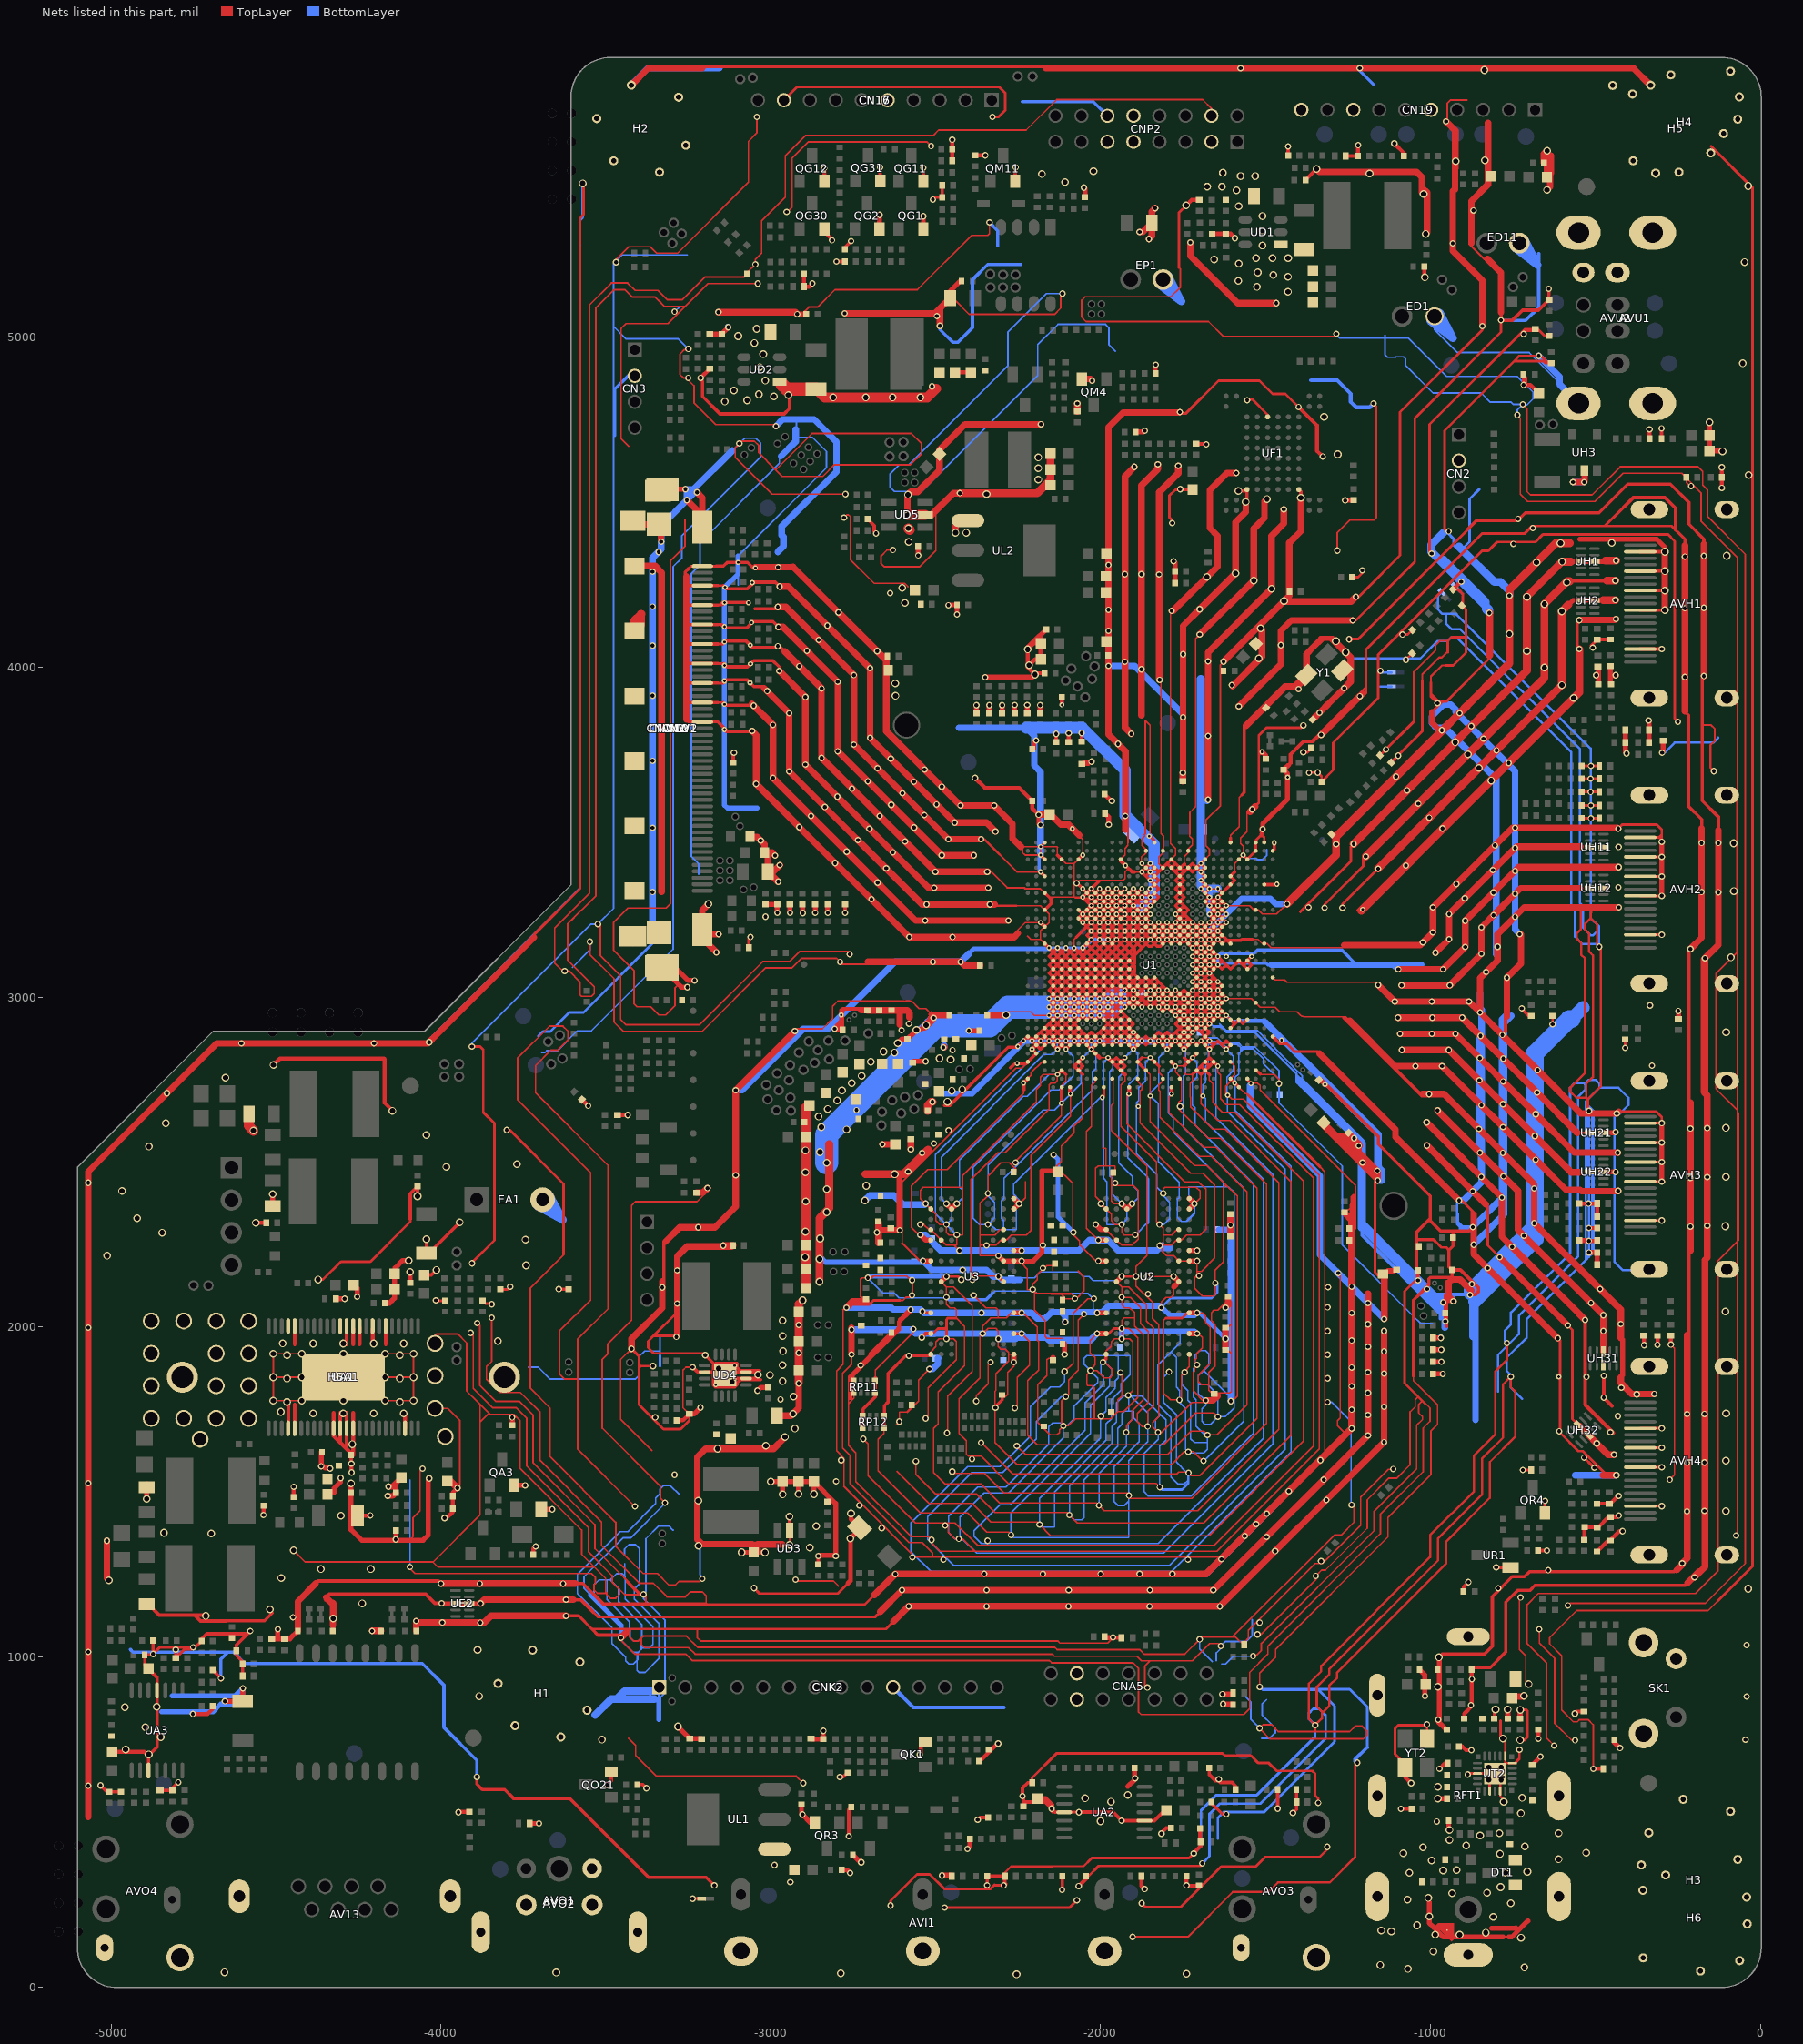
[diagram p0: the nets of this part, all layers, seen from the top]
# Altium PCB MISC86290.PcbDoc (part 18 of 31)
Units mil, origin at the board's own origin, x right, y up, seen from the top; angles counter-clockwise.
Board outline 5104.71 x 5851.49 mil, 2 copper layers (TopLayer, BottomLayer), stack 61.855 mil thick; 1026 components, 667 nets, 4280 pads, 2294 vias.

## Via types
v1: diameter 19.68, hole 11.81, TopLayer to BottomLayer, tented both sides, 1189 vias
v2: diameter 19.68/19.68 (per signal layer), hole 11.81, TopLayer to BottomLayer, tented both sides, 366 vias
v3: diameter 15.75, hole 7.87, TopLayer to BottomLayer, tented both sides, 348 vias
v4: diameter 23.62, hole 15.75, TopLayer to BottomLayer, tented both sides, 309 vias
v5: diameter 15.75/15.75 (per signal layer), hole 7.87, TopLayer to BottomLayer, tented both sides, 59 vias
v6: diameter 24/24 (per signal layer), hole 16, TopLayer to BottomLayer, tented both sides, 23 vias

## Nets (pads, with @x,y where several pads share a name; then routed paths per layer and width w, separated by ;. In a path a pad name is that pad's centre, name@x,y a point inside that pad or via, vN(x,y) a via of type N, cw(c..) or ccw(c..) an arc to the next point about the centre after c; other vN are vias at no path point) (continued)
GND: (continued)
  TopLayer w10: U1.W10@-1708.98,3187.6 v3(-1696.18,3174.8) U1.V9@-1683.39,3162.01 v3(-1670.59,3149.21) U1.U8@-1657.8,3136.42 ; -1696.18,2790.94 U1.C9@-1683.39,2778.15 ; -1696.18,2790.94 U1.D9@-1683.39,2803.74 ; v3(-1696.18,2867.72) U1.F9@-1683.39,2854.92 ; v3(-1696.18,2867.72) -1670.59,2893.31 U1.H9@-1683.39,2906.1 ; -1696.18,2893.31 U1.G9@-1683.39,2880.51 v3(-1670.59,2867.72) ; -1696.18,2893.31 U1.H9@-1683.39,2906.1 ; v3(-1696.18,2918.9) U1.H9@-1683.39,2906.1 ; v3(-1696.18,2918.9) U1.J9@-1683.39,2931.69 ; v3(-1696.18,2944.49) U1.J9@-1683.39,2931.69 ; v3(-1696.18,2944.49) -1683.39,2957.28 ; v3(-1696.18,2970.08) -1683.39,2957.28 ; v3(-1696.18,2970.08) U1.L9@-1683.39,2982.87 v3(-1670.59,2995.67) -1657.8,3008.46 v3(-1645,3021.26) U1.N7@-1632.2,3034.06 v3(-1645,3046.85) ; U1.C9@-1683.39,2778.15 -1670.59,2790.94 ; U1.D9@-1683.39,2803.74 -1670.59,2790.94 ; U1.D9@-1683.39,2803.74 -1670.59,2816.54 U1.D8@-1657.8,2803.74 ; U1.F9@-1683.39,2854.92 v5(-1670.59,2842.13) -1657.8,2854.92 ; U1.F9@-1683.39,2854.92 v3(-1670.59,2867.72) ; U1.H9@-1683.39,2906.1 v3(-1670.59,2918.9) ; U1.J9@-1683.39,2931.69 v3(-1670.59,2918.9) ; U1.J9@-1683.39,2931.69 v3(-1670.59,2944.49) ; -1683.39,2957.28 v3(-1670.59,2944.49) ; -1683.39,2957.28 v3(-1670.59,2970.08) U1.L8@-1657.8,2982.87 v3(-1645,2995.67) U1.M7@-1632.2,3008.46 ; U1.Y9@-1683.39,3213.19 v3(-1670.59,3225.98) ; U1.Y9@-1683.39,3213.19 v3(-1670.59,3200.39) ; U1.AD9@-1683.39,3315.55 v3(-1670.59,3302.76) ; -1670.59,2790.94 U1.D8@-1657.8,2803.74 ; v3(-1670.59,2867.72) -1657.8,2854.92 ; v3(-1670.59,2918.9) U1.J8@-1657.8,2931.69 ; v3(-1670.59,2944.49) U1.K8@-1657.8,2957.28 v3(-1645,2970.08) U1.L7@-1632.2,2982.87 ; v3(-1670.59,2944.49) U1.J8@-1657.8,2931.69 ; v3(-1670.59,3200.39) U1.Y8@-1657.8,3213.19 ; v3(-1670.59,3200.39) U1.W8@-1657.8,3187.6 v3(-1645,3174.8) U1.V7@-1632.2,3162.01 -1619.41,3174.8 ; v3(-1670.59,3225.98) U1.AA8@-1657.8,3238.78 ; v3(-1670.59,3225.98) U1.Y8@-1657.8,3213.19 ; v3(-1670.59,3277.17) U1.AC9@-1683.39,3289.96 v3(-1670.59,3302.76) ; v3(-1670.59,3277.17) v3(-1645,3251.57) ; v3(-1670.59,3277.17) U1.AC8@-1657.8,3289.96 ; v3(-1670.59,3302.76) U1.AC8@-1657.8,3289.96 ; -1657.8,2854.92 -1645,2867.72 -1632.52,2855.24 ; -1657.8,3059.65 v3(-1645,3046.85) ; -1657.8,3059.65 v3(-1721.77,3123.62) U1.Y7@-1632.2,3213.19 ; U1.U8@-1657.8,3136.42 v3(-1721.77,3072.44) U1.L7@-1632.2,2982.87 ; U1.U8@-1657.8,3136.42 v3(-1645,3123.62) ; U1.Y8@-1657.8,3213.19 U1.AA7@-1632.2,3238.78 ; U1.Y8@-1657.8,3213.19 v3(-1645,3200.39) U1.W7@-1632.2,3187.6 ; U1.AA8@-1657.8,3238.78 v3(-1670.59,3251.57) U1.AB8@-1657.8,3264.37 v3(-1645,3277.17) ; U1.AA8@-1657.8,3238.78 v3(-1645,3225.98) U1.Y7@-1632.2,3213.19 ; U1.AA8@-1657.8,3238.78 v3(-1645,3251.57) ; U1.AC8@-1657.8,3289.96 v3(-1645,3277.17) ; U1.AC8@-1657.8,3289.96 v3(-1645,3302.76) ; v3(-1645,3098.03) -1632.2,3085.24 -1619.41,3098.03 ; v3(-1645,3098.03) -1632.2,3110.83 ; v3(-1645,3123.62) -1632.2,3110.83 ; v3(-1645,3251.57) U1.AA7@-1632.2,3238.78 ; v3(-1645,3251.57) U1.AB7@-1632.2,3264.37 ; v3(-1645,3277.17) U1.AC7@-1632.2,3289.96 ; v3(-1645,3277.17) U1.AB7@-1632.2,3264.37 ; v3(-1645,3302.76) U1.AC7@-1632.2,3289.96 ; v3(-1645,3302.76) U1.AD7@-1632.2,3315.55 ; U1.L7@-1632.2,2982.87 -1619.34,2995.74 -1632.07,3008.46 U1.M7@-1632.2,3008.46 ; U1.M7@-1632.2,3008.46 v3(-1721.77,3098.03) U1.W7@-1632.2,3187.6 ; -1632.2,3110.83 -1619.41,3098.03 ; U1.W7@-1632.2,3187.6 -1619.41,3174.8 ; U1.Y7@-1632.2,3213.19 v3(-1619.41,3225.98) U1.AA7@-1632.2,3238.78 ; U1.AA7@-1632.2,3238.78 v3(-1619.41,3251.57) U1.AB7@-1632.2,3264.37 ; U1.AB7@-1632.2,3264.37 v3(-1619.41,3277.17) U1.AC7@-1632.2,3289.96 ; -1619.41,3098.03 -1606.61,3085.24 U1.T5@-1581.02,3110.83 -1568.23,3098.03 ; -1619.41,3174.8 -1617.01,3172.4 -1574.73,3172.4 ; -1568.23,3098.03 U1.T4@-1555.43,3110.83 ; -1568.23,3098.03 U1.R4@-1555.43,3085.24 -1542.64,3098.03 U1.T4@-1555.43,3110.83 ; -944.34,2220 -944.34,2182.31 RO2.1@-935.04,2173 ; -752.48,1243 -715.33,1243 -700.58,1257.75 v1@-638.28,1257.75 ; v1@-731,4450 -712.8,4468.2 -672.72,4468.2
  TopLayer w11: UA1.4@-4463.07,1692.73 pad.VIA5@-4463.07,1769.34 ; UA1.5@-4443.39,1692.73 -4443.39,1765.61 ; v1(-2066,529) -1962.59,529 v1(-1937,503.41) UA2.10@-1867.44,503.41 -1837.59,503.41 -1806,535 CO20.1@-1800.81,535 ; v1(-1816,464) -1816,466 -1801,481 CO21.1@-1786.73,481
  TopLayer w11.8: -4443.39,1947.88 UA1.44@-4443.39,1994.89 ; -4325.28,1739.74 -4325.28,1669.55 -4272.48,1616.75 CA7.1@-4272.48,1611.81 -4272.48,1586.54 v1(-4271.75,1585.81) -4271.75,1559.31 v1(-4271.25,1558.81) ; -4305.59,1651.81 v4@-4305.59,1739.74 ; -4285.91,1634.31 v4@-4285.91,1739.74 ; v4@-4285.91,1947.88 UA1.36@-4285.91,1994.89 ; CA7.1@-4266.22,1611.31 -4266.22,1739.74 ; -4266.22,1947.88 UA1.35@-4266.22,1994.89 ; -4246.54,1947.88 UA1.34@-4246.54,1998.83 ; v4@-4207.17,1947.88 UA1.32@-4207.17,1994.89 ; -4167.8,1947.88 UA1.30@-4167.8,1994.89 ; UA1.22@-4108.74,1692.73 v4@-4108.74,1739.74
  TopLayer w11.81: -2233.58,2719.09 v5(-2233.58,2739.76) U1.B30@-2220.79,2752.56 ; v5@-2118.43,2679.72 U1.A26@-2118.43,2726.97 ; v5@-2092.83,2706.3 U1.A25@-2092.83,2726.97 ; v5@-2028.76,2842.03 U1.E22@-2016.06,2829.33 -2003.27,2816.54 ; v5(-1977.68,2816.54) U1.D20@-1964.88,2803.74 ; U1.D19@-1940.28,2802.76 U1.D19@-1939.29,2803.74 ; U1.C19@-1939.29,2778.15 -1926.5,2765.35 ; v5(-1914.69,2706.3) -1913.7,2707.28 U1.A18@-1913.7,2726.97 ; U1.AD16@-1862.52,3315.55 v3(-1849.72,3302.76) ; v5(-1785.75,2706.3) U1.A13@-1785.75,2726.97 ; U1.D13@-1785.75,2803.74 v5(-1772.95,2790.94)
  TopLayer w12: CO36.1@-4997,711.81 -4899.06,711.81 v4@-4887.25,700 ; v1(-4752,827) -4707.5,827 -4691.78,842.72 CA56.1@-4691.78,851 ; v4(-4561.77,2316.01) CA34.2@-4529.5,2316.01 ; v1(-4538,1430) -4537.39,1430.61 CA33.2@-4537.39,1457.79 ; v4(-4508,2794) -4488.11,2813.89 -4171.88,2813.89 -4170.5,2812.51 -4170.5,2679 v4(-4147,2655.5) ; CA32.2@-4446.39,1484.25 v1(-4446.39,1515.52) ; -4348.5,1173 -4348.5,1180 -4338.5,1190 -4046.26,1190 -4018.56,1162.29 v1(-3997.99,1162.29) -3997.7,1162 UE2.GND@-3955.47,1162 v1(-3880,1162) ; CA31.1@-4253.33,1427.57 -4215.43,1427.57 v1(-4214,1429) ; v1(-3989,1421) -3988.04,1420.04 -3983.04,1420.04 -3964.27,1438.82 RA15.2@-3964.27,1450 CA20.2@-3964.27,1487 -3964.27,1498.08 v1@-3950.35,1512 ; v1(-3947,529) -3946,530 CO2.1@-3914.25,530 ; RA26.1@-3719.73,1310 -3719.73,1328.27 v1(-3713,1335) ; RW4.1@-3572.67,2689.67 v1(-3553.5,2670.5) ; D4.A@-3465,2642.73 v1(-3433.73,2642.73) ; CNW1.53@-3342.82,3094.05 CNW1.53@-3330.77,3082 ; RD33.1@-3285.27,1717 -3266.52,1717 CD34.1@-3247.25,1736.27 ; v1@-3215.25,4875 RD16.1@-3185.25,4905 v1(-3212.75,4877.5) ; UD3.2@-2943.25,1383.12 v4(-2943.25,1425.25) ; RG31.1@-2899.27,5192 DG1.A@-2899.27,5154 -2883.5,5154 v1(-2874,5163.5) ; DK9.A@-2877.74,749.27 -2842.48,749.27 CK9.1@-2840.75,751 v1(-2840.75,775.75) ; RD23.1@-2856.25,1279.73 v1(-2856.25,1305.75) ; QG30.E@-2837.81,5329 -2837.81,5320.81 -2814.5,5297.5 v1(-2814.5,5294.5) ; QG12.E@-2837.81,5473.12 v1(-2837.81,5512.81) ; v1(-2801,5230) CG30.1@-2775.73,5230 ; v1@-2799.96,2903 -2799.96,2914.61 ; -2789.16,2925.42 -2799.96,2914.61 ; -2785,2959.5 -2780,2964.5 ; C6.2@-2781.96,2900.5 -2796.08,2914.61 -2799.96,2914.61 ; -2781.5,2963 -2780,2964.5 ; v1(-2775,3256) RW414.1@-2775,3281.27 ; C11.1@-2707.95,2960.5 -2711.95,2964.5 -2780,2964.5 ; QG31.E@-2668.5,5477 v1(-2668.5,5515.5) ; v1(-2548.84,703.8) -2545,707.64 -2545,728.5 QK1.E@-2532.5,741 ; QG11.E@-2537.75,5476.12 v1(-2537.75,5514.25) ; RG14.1@-2450.27,5535.5 CG11.1@-2450.27,5570.5 v1(-2450.27,5599.23) ; CD17.1@-2441.75,4894.19 CD18.1@-2393.75,4894.19 ; v1(-2381,3664.61) -2350.5,3634.11 -2246.73,3634.11 C26.2@-2207.73,3595.11 -2207.73,3572.01 -2188.98,3553.26 v1@-2185.15,3553.26 ; RM12.1@-2381,5552.23 v1(-2349.77,5552.23) ; CK8.1@-2368.27,684 -2366.04,684 v1@-2313.04,737 ; QM11.E@-2259.25,5473.13 v1@-2259.25,5513.75 ; v4(-2217,4006) -2199,4024 C35.1@-2181.81,4024 ; v4@-2202,3982 C33.2@-2170.73,3982 ; R8.1@-2201.73,3752 -2201.73,3772.27 v1(-2196,3778) ; v4(-2199,3978) -2221,4000 v4(-2221,4054) ; v1(-2188,3553) -2188,3523.6 -2186.4,3522 v1(-2182.5,3522) ; -2187.47,4095.97 -2221,4062.44 v4(-2221,4054) ; v3(-2182.4,3225.98) U1.Y28@-2169.61,3213.19 ; C36.1@-2181.81,4072 -2203,4072 v4(-2221,4054) ; R9.1@-2135,3772.73 v1(-2135,3798) ; C32.2@-2117.73,3909 -2117.73,3886.23 v3(-2117.5,3886) ; R24.1@-2097,3772.73 v1(-2097,3800) ; v1(-2067,305.09) CI3.1@-2043.54,328.55 ; R25.1@-2058,3774.73 v1(-2058,3801) ; -2037.27,3706.73 R27.1@-2057,3706.73 -2049.73,3714 v1(-2028,3714) ; R11.1@-1988.27,3615 -1967.27,3594 -1967,3594 v1(-1966,3595) ; -1974,1058 DA5.A@-1936.73,1058 ; DI3.A@-1876.27,335 -1876.27,305.27 v1(-1867,296) ; CM1.1@-1833.33,4891 v1(-1833.33,4917.33) ; v4(-1741,5400) -1724.27,5416.73 RD6.1@-1701.25,5416.73 ; RI5.1@-1740.27,336 v1@-1740.27,307.19 ; v1(-1740.16,307.09) v1@-1740.27,307.19 ; v1(-1718,404) -1718,405.48 -1697.73,425.74 DO12.A@-1697.73,440 -1698.73,441 RO25.1@-1698.73,480 ; RD6.1@-1702.04,5418.73 RD6.1@-1701.25,5418.73 ; CI5.1@-1702,306.27 -1739.34,306.27 v1@-1740.27,307.19 ; CD4.2@-1621.02,5313.27 -1605.52,5313.27 v1(-1593.25,5301) ; CT12.1@-1445.5,3689.27 -1444.71,3689.27 -1424.66,3709.32 -1424.66,3735.35 -1384.73,3775.28 -1357.09,3775.28 v1@-1337.37,3795 ; CU11.2@-1431.73,5551 v1(-1431.73,5578.73) ; v1(-1400.18,4789.18) -1344.75,4733.75 -1344.75,4656.75 ; CD2.1@-1379.27,5477 -1346,5510.27 v4(-1346,5511) ; -1344.75,4655.75 -1344.75,4656.75 ; v1(-1327,4639) -1344.75,4656.75 ; DW1.A@-1257.27,5550 -1219.73,5550 v1(-1219.73,5582.73) ; v1(-1110,5588) -1080.62,5558.62 CU13.2@-1080.62,5550.24 ; YT2.2@-1077.46,664.69 -1077.46,635.46 v1(-1059,617) ; v4@-1019.27,5184.27 CD7.1@-1019.27,5215 ; v1(-973.04,660.69) -955.86,677.86 CT40.1@-949.11,677.86 ; RO53.1@-932.74,4235.43 -908.88,4259.29 v1(-906.89,4259.29) ; CT39.1@-914.18,728.42 -903.97,728.42 -892.67,717.12 v1(-876.18,717.12) ; CT8.1@-897.82,813.34 -897.82,827.95 ; v1(-877.82,853.61) -877.82,847.95 -897.82,827.95 ; CT21.2@-875.09,961.61 v1(-875.09,932.61) -875.09,850.68 -897.82,827.95 ; CT20.1@-806.03,813.16 v4@-806.03,836.66 ; CU4.1@-717.73,4888 v1@-717.73,4856 ; v1@-712.73,4857.27 -712.73,4878 ; CT5.2@-692,672.23 v1(-667,697.23) ; v1(-673,752) CT10.1@-673,779.27 ; CU3.1@-671,4829.81 -697.19,4856 v1@-717.73,4856 ; v1(-562.5,828) -556.23,834.27 CR3.1@-535,834.27 ; CH24.2@-548.27,2374 v1@-523,2374 ; CH32.2@-534,1354.73 -534,1392.27 CH33.2@-533,1393.27 -497,1393.27 DH33.A@-495,1391.27 -493.22,1391.27 -460.76,1423.73 v2@-434.93,1423.73 ; v1@-531.38,2021.61 -531.38,1805 ; v1(-527.54,1848.6) -531.38,1844.75 -531.38,1805 ; v1(-520,2261) DH22.A@-494.73,2261 ; v1(-520,2300) CH23.2@-494.73,2300 ; v1@-519.02,2374 DH24.A@-494.73,2374 ; CH31.2@-496,1319.54 -495.21,1319.54 -462.01,1352.73 DH32.A@-456,1352.73 -427.73,1381 v2(-418,1381) ; CH34.2@-496,1464.27 DH34.A@-458,1464.27 -454.98,1464.27 -431.25,1488 v2(-430,1488) ; DH23.A@-494.73,2334 DH24.A@-494.73,2374 ; DH24.A@-493.75,2374 DH24.A@-494.73,2374 ; v1(-475,1852) v1(-475,1786) -450,1761 ; v2@-446,1679 -531.38,1764.38 -531.38,1805 ; v1(-352.5,1945) DH35.A@-352.5,1972.77 ; RU3.2@-336.27,4693 v1(-336.27,4721.27) ; v1(-312,1946) CH15.1@-312,1973.27 ; v1(-300,4724.39) -299.73,4724.12 CU1.2@-299.73,4693 ; v1(-271.5,1946.5) DH36.A@-271.5,1973.77 ; v1(-117.27,4543.73) DT3.A@-117.27,4576 v1(-117.27,4606.27) ; v1@-717.73,4856 -717.73,4855.27 -718,4855.54 v1(-718,4856) v1@-717.73,4856
  TopLayer w14: -582,4189 -568.63,4202.37 UH2.GND@-503.25,4202.37 -477.78,4202.37 ; -575.25,4320.31 UH1.GND@-544.19,4320.31 UH1.GND@-503.25,4320.31 -472.29,4320.31
  TopLayer w15: v4@-4892.03,1488.03 CA17.2@-4892.03,1524.03 ; v1(-4655,865.5) -4654.94,865.56 CE5.2@-4601.05,865.56 -4601.05,904.45 v1(-4600.5,905) ; CE6.2@-4513.06,1054.71 -4494.5,1054.71 ; CA26.2@-4510.33,2366.98 v4(-4510.33,2402.45) ; v1(-4494.5,1084) -4494.5,1054.71 ; CE4.1@-4433.73,1078.79 -4457.81,1054.71 -4494.5,1054.71 ; CA2.1@-4363.02,1620.81 -4363.02,1584.8 -4350.53,1572.31 -4337.25,1572.31 v1(-4336.25,1571.31) ; -4324.22,1498.31 -4324.22,1510.34 -4304.25,1530.31 v1(-4304.25,1542.31) ; CA8.1@-4318.77,2085.5 v1(-4292,2085.5) ; v4@-4272.48,1525.48 RA8.1@-4272.48,1497.81 -4272.48,1385.48 -4240.66,1353.66 -4096,1353.66 -4054.25,1353.66 -4038.5,1369.4 -4038.5,1538.5 v1(-4036,1541) ; CA6.1@-4264.69,2127.5 -4254,2116.81 v1(-4254,2092) ; CA6.1@-4258.19,2117.19 CA6.1@-4258.19,2135 ; CA23.2@-4170.27,2072 -4156,2072 ; -4145.53,2083.53 -4145.53,2082.47 -4156,2072 ; CA12.1@-4140.69,2161 -4140.69,2087.31 -4156,2072 ; -4140.19,2087.81 CA25.2@-4140.19,2117 ; CA12.1@-4139.19,2166.64 -4139.19,2178.81 -4116.5,2201.5 v4(-4098,2201.5) ; v1(-4137,1356) -4136.73,1356.27 RA7.2@-4136.73,1383 ; v4(-4094,2166.64) -4093,2165.64 CA9.1@-4093,2133.73 ; RA20.1@-3784,1701.73 v1(-3784,1726) ; QA3.E@-3777.5,1520 v1(-3745,1520) ; DO1.A@-3731.52,495 v1(-3703,495) ; CA36.1@-3695.97,1447 v1(-3663,1447) ; CNW1.52@-3342.82,4535 -3337.82,4540 v1(-3259,4540) ; v4(-3282,788.81) DK10.A@-3245.92,752.72 CK3.1@-3211.64,752.72 ; v1@-3253.5,3030.5 -3271.5,3030.5 -3328.73,3087.73 CNW12.61@-3328.73,3090.12 -3290.12,3090.12 -3250.5,3050.5 v1(-3231,3050.5) ; CD34.1@-3247.25,1736.27 -3232.98,1736.27 v1(-3213.25,1756) ; RD12.1@-3185,5009.73 CD29.2@-3149,5009.73 -3149,5010.69 v1(-3128.92,5030.76) ; v4(-3088.81,1316.81) CD21.1@-3052,1316.81 v4(-3017.81,1316.81) ; v1(-3040.5,1807) -3030.27,1817.23 CD30.1@-3007.5,1817.23 ; RW389.1@-3016.5,3281 RW412.1@-2980.7,3281 ; v4(-3000.06,1531.06) CD25.1@-2963.9,1531.06 ; v1@-2989.25,369.25 v1(-2989,369) ; UL1.1@-2989.25,416.9 UL1.1@-2957.9,416.9 ; v1(-2980.5,3256) RW412.1@-2980.5,3280.8 ; v4(-2963.9,1492.1) CD25.1@-2963.9,1531.06 ; RW413.1@-2942.5,3280.8 -2942.5,3257 v1(-2941.5,3256) ; v1(-2920,5070.5) CD12.1@-2892.23,5070.5 ; v4(-2916.59,1493.59) CD26.1@-2916.59,1531.06 ; v1(-2915.57,1921.43) C63.1@-2915.57,1956.38 ; v1(-2915.57,2006.43) C62.1@-2915.57,2045.13 ; CL1.2@-2907.25,552.27 -2907.25,525.25 v1(-2904,522) -2879,497 QR3.E@-2866.75,497 ; RW417.1@-2904.34,3280.53 -2904.34,3255.84 v1(-2903.5,3255) ; v1@-2903.34,3257 RW417.1@-2903.34,3280.53 ; v4(-2869.29,1493.29) CD27.1@-2869.29,1531.06 ; v1(-2865.5,3256) RW252.1@-2865.5,3280.8 ; v1@-2854,1308 -2805.25,1308 v1(-2803.25,1306) -2803.25,1465.02 CD27.1@-2869.29,1531.06 ; v1(-2827.5,3255.83) RW416.1@-2827.5,3280.53 ; v1@-2805.43,2905.26 -2785,2925.7 ; v1@-2799.96,2903 -2797.46,2900.5 C6.2@-2781.96,2900.5 -2785,2903.54 pad.VIA5@-2785,2947.5 ; CL3.2@-2785.52,354.33 -2769.33,354.33 v1(-2760,345) ; -2785,2934.53 pad.VIA5@-2785,2947.5 ; -2781.5,2963 -2785,2959.5 pad.VIA5@-2785,2947.5 ; -2766,1223 -2758.25,1230.75 v4@-2758.25,1359.75 ; -2759.72,1786.37 -2759.72,1848.03 v2@-2727.68,1880.08 ; v4(-2759,1359) v4@-2758.25,1359.75 ; v4@-2758.25,1360.19 v4@-2758.25,1359.75 ; v4(-2757,1434.53) -2757,1418 DD2.A@-2730.54,1391.54 -2730.54,1387.46 v4@-2758.25,1359.75 ; RR16.1@-2751.52,400 -2728.52,377 v1(-2726,377) ; v2@-2727.68,1880.97 -2694.72,1913.93 ; QG2.E@-2670.5,5329 v1(-2670.5,5371.5) ; v4(-2615,2860.5) -2602.45,2873.05 C38.2@-2585.66,2873.05 -2565.15,2893.56 -2565.15,2899.85 -2547.15,2899.85 v6@-2535.5,2911.5 ; -2607.06,2021.8 v2(-2576.1,2052.76) ; C45.2@-2570,2801.5 -2566,2805.5 v1(-2531,2805.5) ; v1(-2553.23,4338.97) CD52.2@-2553.23,4366.23 ; QG1.E@-2537.75,5329 v1(-2537.75,5367.25) ; -2481.28,5094 CM17.2@-2456.28,5119 -2456.28,5140.22 -2425.5,5171 RM15.2@-2421.98,5171 ; v1(-2481,337) -2479.16,338.84 DI1.A@-2451.73,338.84 ; v1(-2462,4188) -2460.89,4189.11 CL55.1@-2435.73,4189.11 v1(-2435.73,4160.27) ; v1(-2404,418) -2396.46,425.54 RO20.1@-2396.46,448 ; v1(-2400.03,2898.03) R49.1@-2367.19,2898.03 ; v1@-2376.75,3883.83 R21.1@-2376.75,3860.3 v1(-2376.75,3885) ; v1@-2352,3970 -2207,3970 v4(-2199,3978) ; R26.1@-2338.63,3859.41 v1@-2338.63,3884.11 ; v1@-2337.75,3883.83 R26.1@-2337.75,3860.3 v1(-2337.75,3885) ; v1@-2298.75,3883.83 R23.1@-2298.75,3860.3 v1(-2298.75,3885) ; v1(-2294,307.09) v1@-2290.73,310.35 ; v1(-2260.82,3885.66) -2260.75,3885.59 R20.1@-2260.75,3860.3 v1@-2260.75,3883.83 ; v2@-2238.13,2199.03 -2204.72,2199.03 -2178.72,2225.03 -2178.72,2473.31 C51.1@-2134.76,2473.31 ; R22.1@-2222.75,3860.3 -2222.75,3870.11 ; v1@-2222.75,3883.83 -2222.75,3870.11 ; v1(-2222.75,3885.95) -2222.75,3870.11 ; CO17.2@-2191,569.81 -2167.15,569.81 -2148.66,551.32 v1(-2148.66,539.86) ; v1(-2188,3553) -2187.74,3553.26 -2153.63,3553.26 v1@-2185.15,3553.26 ; v1@-2183.75,3884.06 R10.1@-2183.75,3860.53 v1(-2183.75,3885.23) ; C35.1@-2181.81,4024 -2181.81,4095.19 ; C36.1@-2181.81,4072 -2181.81,4097.92 C34.2@-2165.23,4114.5 ; v1(-2117,294) v1@-2116.54,294.46 ; v1(-2051,5454) -2048,5451 CP2.1@-2048,5425.73 ; DA6.A@-1988.27,1058 -1974,1058 ; DR5.A@-1987.27,3557.11 -1976,3545.84 v1(-1976,3523.11) ; -1918,606.67 -1895.5,629.17 v1(-1895.5,632) ; v1@-1897.77,634.27 CO15.1@-1897.77,663 ; RF1.1@-1893.78,4713.11 -1870.46,4713.11 v1(-1866.46,4717.11) ; v1(-1778.99,4321.51) -1774.73,4317.25 C23.2@-1774.73,4291 C22.2@-1774.73,4255 ; RD2.1@-1662.25,5314.27 -1606.52,5314.27 -1605.52,5313.27 ; v1(-1631,887) -1602.73,887 DA1.A@-1598.73,891 ; v1(-1629,857) -1600.73,857 CA29.1@-1598.73,855 ; -1511.29,3491.86 -1511.29,3493.82 ; v1@-1511.29,3503.11 -1511.29,3511.03 v1@-1509,3513.32 ; v3(-1510.98,3743.7) -1499.5,3732.22 CT14.2@-1499.5,3721.96 ; v1(-1509,3509.11) v1@-1509,3513.32 ; v3(-1433.5,3666.5) -1433.5,3600.87 ; -1433.25,3701.37 -1445.36,3689.27 CT12.1@-1445.5,3689.27 -1433.5,3677.27 -1433.5,3600.87 ; C111.1@-1338.32,2749.32 -1334.55,2749.32 v3(-1320.46,2735.22) ; -1333.04,4087.61 -1299.61,4087.61 -1297.11,4085.11 ; -1308.35,2598.65 -1290.7,2581 -1256.84,2581 C24.2@-1248.67,2589.17 -1231.9,2572.4 -1217.82,2558.32 v1(-1217.82,2549.62) ; v1@-1257.7,4506.77 CF2.1@-1233,4506.77 ; -1235.75,2370.84 -1235.75,2393.03 -1233.25,2395.53 ; CT33.1@-1033.27,961 -1017,944.73 v1(-1017,881) ; -1004.03,256.5 v4(-1004.03,212.86) -1004.03,193.5 -991.1,180.57 -990.97,180.44 -979.12,168.59 -961.43,150.9 -780.03,150.9 ; C14.2@-993,1857.84 v1(-963.16,1857.84) ; C15.2@-993,1894.56 v1(-967.06,1894.56) ; C27.2@-993,1931 v1(-967.5,1931) ; C28.2@-993,1967 v1(-969,1967) ; v4@-978.03,609.65 v4@-973.53,605.15 ; v1(-976.82,809.61) -976.82,802.96 CT7.1@-953.73,779.87 ; v4@-973.16,991.7 -973.16,799.3 CT7.1@-953.73,779.87 ; v4@-969.03,570.15 CT1.1@-949.76,570.15 ; CT7.1@-950.82,779.87 CT7.1@-953.73,779.87 ; CT2.1@-945.09,503.15 -945.09,477.72 v4(-942.53,475.15) ; -814.84,177.5 -742.3,177.5 -741.03,178.77 ; -762.47,150.5 -754.14,150.5 -705.03,199.61 ; CH21.2@-549.27,2262 -521,2262 v1(-520,2261) ; -547.8,4387.7 -313.7,4387.7 -289.88,4363.88 v4(-289.88,4350.4) ; v1@-519.68,2226 CH22.2@-494.73,2226 DH21.A@-494.73,2189 ; v1@-500,3976 v1(-498,3976) v1@-491,3976 ; CH5.2@-491,3948.73 v1@-491,3976 ; DH4.A@-491,4000.27 v1@-491,3976 ; UH22.GND@-475.53,2470 v1(-439,2470) ; UH21.GND@-475.53,2589 -441,2589 v1(-439,2591) ; CH4.2@-455,3950.73 -455,3975 ; DH3.A@-455,4003 -455,3975 ; CR4.1@-442.77,748.5 -442.77,740.27 v1(-426,723.5) ; v1(-439.15,3976) -438,3976 -437,3975 -455,3975 ; -417.76,1853.74 -417.76,1961.06 ; DH2.A@-409.27,3810 -409.27,3742.27 v1(-406,3739) ; v1(-339,3839) -337.27,3837.27 CH1.2@-337.27,3772 ; v2(-299,2618) -299,2443.29 v2@-296.66,2440.95 ; v1(-299,3471) -299,3310.04 v2@-296.05,3307.09 ; v1(-298,3741) -295,3744 CH16.1@-295,3777.27 ; v1(-249,2958) -248.64,2957.64 DH37.A@-248.64,2933.96 ; v4(-154,4743) -154.19,4742.81 CU5.2@-154.19,4703 -154.19,4656 v4@-116,4656 ; CD25.1@-2963.9,1531.06 CD26.1@-2916.59,1531.06 ; CD26.1@-2916.59,1531.06 CD27.1@-2869.29,1531.06 ; v1@-1509,3513.32 -1509,3525.15 -1494.63,3539.52 -1494.63,3539.74 -1433.5,3600.87
  TopLayer w15.75: v2@-2610.81,2292.91 -2610.81,2463.03 ; v2(-2546.57,2279.13) -2530.83,2263.39 U3.E1@-2515.08,2263.39 ; v2(-2538.7,2200.39) U3.G1@-2515.08,2200.39 ; U3.J2@-2483.58,2137.4 v2(-2467.83,2153.15) ; v2(-2467.83,2373.62) U3.B3@-2452.09,2357.87 v2(-2436.34,2373.62) ; v2(-2310.35,2216.14) U3.G8@-2294.61,2200.39 v2(-2239.49,2200.39) ; v2(-2263.11,1893.31) U3.T9@-2263.11,1916.93 ; U3.M9@-2263.11,2042.91 v2(-2239.49,2042.91) ; U3.F9@-2263.11,2231.89 v2(-2239.49,2231.89) ; U3.B9@-2263.11,2357.87 v2(-2247.36,2373.62) U3.A9@-2263.11,2389.37 ; C42.2@-2145,1905.43 C42.2@-2145,1907.11 ; v2@-2109.25,1917.24 R108.1@-2109.25,1948.43 ; v2(-2015.08,2310.63) -1999.33,2294.88 U2.D1@-1983.58,2294.88 ; v2(-2011.14,1979.92) U2.P1@-1983.58,1979.92 ; v2(-2011.14,2042.91) U2.M1@-1983.58,2042.91 ; v2(-2007.2,2200.39) U2.G1@-1983.58,2200.39 ; v2(-2007.2,2263.39) U2.E1@-1983.58,2263.39 ; U2.J2@-1952.09,2137.4 v2(-1936.34,2153.15) ; v2(-1936.34,2373.62) U2.B3@-1920.59,2357.87 v2(-1904.84,2373.62) ; -1778.86,2121.65 U2.J8@-1763.11,2137.4 v2(-1778.86,2153.15) ; U2.P9@-1731.61,1979.92 v2(-1707.99,1979.92) ; U2.M9@-1731.61,2042.91 v2(-1707.99,2042.91) ; U2.G9@-1731.61,2200.39 v2(-1707.99,2200.39) ; U2.F9@-1731.61,2231.89 v2(-1707.99,2231.89) ; U2.B9@-1731.61,2357.87 v2(-1715.87,2373.62) U2.A9@-1731.61,2389.37
  TopLayer w17: v1(-4161.25,1487.81) -4146.48,1487.81 CA15.1@-4136.48,1497.81 -4137.59,1498.92 -4137.59,1526.15 ; v1(-4159.27,1516.12) -4147.62,1516.12 -4137.59,1526.15 ; CA16.1@-4119.75,1544 -4137.59,1526.15 ; CT16.1@-766.03,812.88 v4@-766.03,839.65 ; CT17.1@-728.39,812.83 v4@-728.39,839.29
  TopLayer w18: -995.5,3864.77 -995.5,3831.78 -971.72,3808 v1@-965,3808
  TopLayer w19: v2(-1621.38,2058.66) -1613.5,2066.54 R64.1@-1613.5,2085.91
  TopLayer w19.68: v2(-2755.24,1916.93) v2@-2755.24,1998.03 ; C102.1@-2711.21,2078.03 C102.1@-2710.89,2078.35